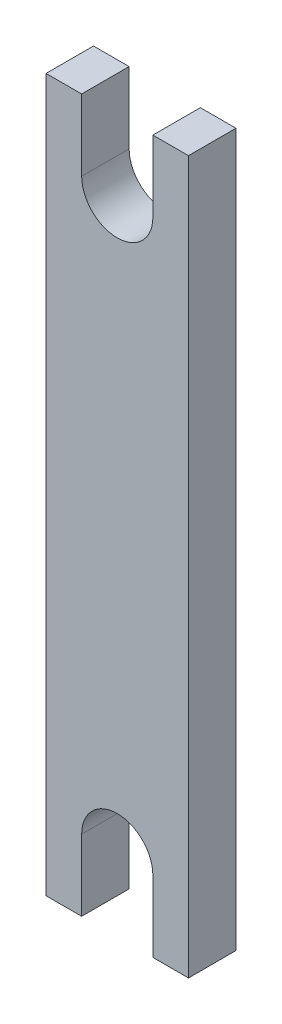
from build123d import *

# Parameters (mm, degrees)
BOSS_EXTRUDE1_DEPTH = 2


with BuildPart() as part:
    # Sketch1 → Boss-Extrude1 (new body)
    with BuildSketch(Plane.XY):
        with BuildLine():
            Line((3, 15), (3, -15))
            Line((3, -15), (1.5, -15))
            Line((1.5, -15), (1.5, -12))
            ThreePointArc((1.5, -12), (0, -10.5), (-1.5, -12))
            Line((-1.5, -12), (-1.5, -15))
            Line((-1.5, -15), (-3, -15))
            Line((-3, -15), (-3, 15))
            Line((-3, 15), (-1.5, 15))
            Line((-1.5, 15), (-1.5, 12))
            ThreePointArc((-1.5, 12), (0, 10.5), (1.5, 12))
            Line((1.5, 12), (1.5, 15))
            Line((1.5, 15), (3, 15))
        make_face()
    extrude(amount=BOSS_EXTRUDE1_DEPTH)


solid = part.part
